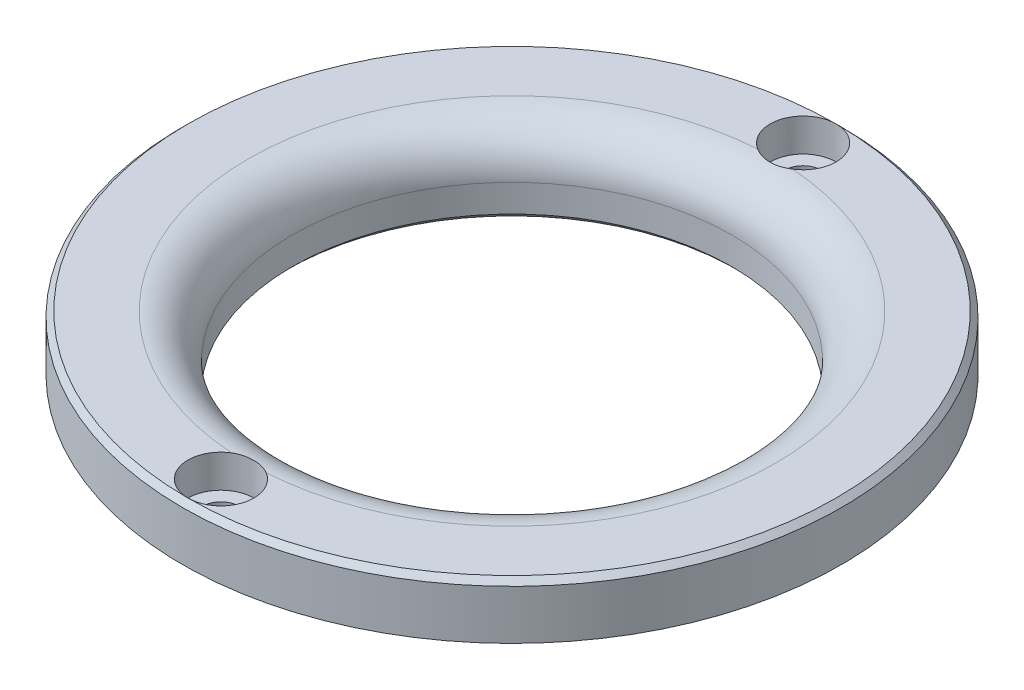
from build123d import *

# Parameters (mm, degrees)
SKETCH1_R                                            = 30
SKETCH1_R_2                                          = 20
BOSS_EXTRUDE1_DEPTH                                  = 3.5
SKETCH2_OUTSIDE_W                                    = 79.028
SKETCH2_OUTSIDE_H                                    = 79.028
SKETCH2_OUTSIDE_R                                    = 23
CUT_EXTRUDE1_DEPTH                                   = 2
FILLET1_R                                            = 4
CHAMFER1_SIZE                                        = 0.5
HOLE_SIZE_BY_SOCKET_HEAD_CAP_SCREW_TYPE1_D           = 3.4
HOLE_SIZE_BY_SOCKET_HEAD_CAP_SCREW_TYPE1_CBORE_D     = 6
HOLE_SIZE_BY_SOCKET_HEAD_CAP_SCREW_TYPE1_CBORE_DEPTH = 3


with BuildPart() as part:
    # Sketch1 → Boss-Extrude1 (new, symmetric)
    with BuildSketch(Plane(origin=(0, 0, 0), x_dir=(1, 0, 0), z_dir=(0, 1, 0))):
        with Locations(Location((0, 0, 0), (0, 0, 270))):
            Circle(SKETCH1_R)
        with Locations(Location((0, 0, 0), (0, 0, 270))):
            Circle(SKETCH1_R_2, mode=Mode.SUBTRACT)
    extrude(amount=BOSS_EXTRUDE1_DEPTH, both=True)

    # Sketch2 outside → Cut-Extrude1 (cut)
    with BuildSketch(Plane.XZ.offset(3.5)):
        Rectangle(SKETCH2_OUTSIDE_W, SKETCH2_OUTSIDE_H)
        with Locations(Location((0, 0, 0), (0, 0, 270))):
            Circle(SKETCH2_OUTSIDE_R, mode=Mode.SUBTRACT)
    extrude(amount=-CUT_EXTRUDE1_DEPTH, mode=Mode.SUBTRACT)

    # Fillet1
    fillet1_edges = [part.edges().sort_by_distance(p)[0] for p in [
        (0, 3.5, -20),
    ]]
    fillet(fillet1_edges, radius=FILLET1_R)

    # Chamfer1
    chamfer1_edges = [part.edges().sort_by_distance(p)[0] for p in [
        (0, -3.5, 23),
        (0, 3.5, -30),
        (0, -3.5, -20),
    ]]
    chamfer(chamfer1_edges, length=CHAMFER1_SIZE)

    # Hole Size by Socket Head Cap Screw Type1 (through all)
    with Locations(Plane(origin=(0, 3.5, 0), x_dir=(1, 0, 0), z_dir=(0, 1, 0))):
        with Locations((0, -26.5), (0, 26.5)):
            CounterBoreHole(HOLE_SIZE_BY_SOCKET_HEAD_CAP_SCREW_TYPE1_D / 2, HOLE_SIZE_BY_SOCKET_HEAD_CAP_SCREW_TYPE1_CBORE_D / 2, HOLE_SIZE_BY_SOCKET_HEAD_CAP_SCREW_TYPE1_CBORE_DEPTH)


solid = part.part
